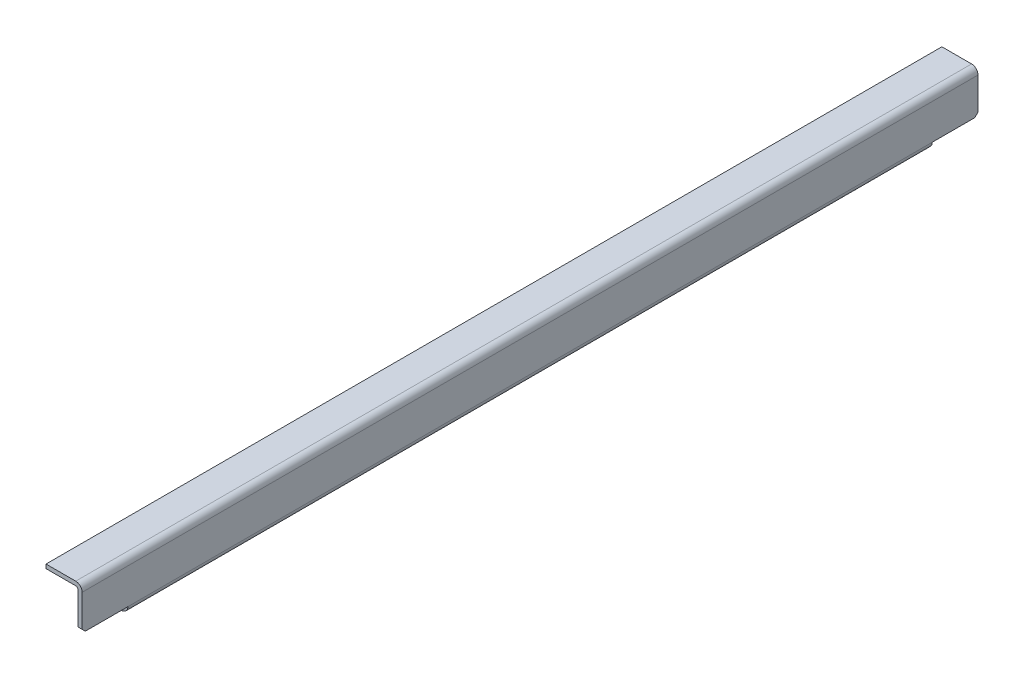
from build123d import *

# Parameters (mm, degrees)
BOSS_EXTRUDE1_DEPTH    = 1116
SKETCH2_W              = 92.475127077
SKETCH2_H              = 38.646657261
SKETCH2_W_2            = 90.397253408
SKETCH2_H_2            = 44.857464027
CUT_EXTRUDE1_DEPTH     = 1116
SKETCH3_R              = 4
CUT_EXTRUDE2_DEPTH     = 1116
M10_TAPPED_HOLE1_D     = 8.5
M10_TAPPED_HOLE1_DEPTH = 24.5
M10_TAPPED_HOLE1_TIP   = 2.553657631
CHAMFER1_SIZE          = 4


with BuildPart() as part:
    # Sketch1 → Boss-Extrude1 (new body)
    with BuildSketch(Plane.XY):
        with BuildLine():
            Line((0, 0), (37, 0))
            ThreePointArc((37, 0), (42.656854249, -2.343145751), (45, -8))
            Line((45, -8), (45, -52))
            ThreePointArc((45, -52), (42.656854249, -57.656854249), (37, -60))
            Line((37, -60), (0, -60))
            Line((0, -60), (0, -55))
            Line((0, -55), (37, -55))
            ThreePointArc((37, -55), (39.121320344, -54.121320344), (40, -52))
            Line((40, -52), (40, -8))
            ThreePointArc((40, -8), (39.121320344, -5.878679656), (37, -5))
            Line((37, -5), (0, -5))
            Line((0, -5), (0, 0))
        make_face()
    extrude(amount=BOSS_EXTRUDE1_DEPTH)

    # Sketch2 → Cut-Extrude1 (cut)
    with BuildSketch(Plane.ZY):
        with Locations((1105.237563539, -71.323328631)):
            Rectangle(SKETCH2_W, SKETCH2_H)
        with Locations((11.801373296, -74.428732013)):
            Rectangle(SKETCH2_W_2, SKETCH2_H_2)
    extrude(amount=-CUT_EXTRUDE1_DEPTH, mode=Mode.SUBTRACT)

    # Sketch3 → Cut-Extrude2 (cut)
    with BuildSketch(Plane(origin=(0, -55, 0), x_dir=(1, 0, 0), z_dir=(0, 1, 0))):
        with Locations(Location((12.5, -92, 0), (0, 0, 270))):
            Circle(SKETCH3_R)
    extrude(amount=-CUT_EXTRUDE2_DEPTH, mode=Mode.SUBTRACT)

    # M10 Tapped Hole1
    with Locations(Plane(origin=(0, -55, 0), x_dir=(1, 0, 0), z_dir=(0, 1, 0))):
        with Locations((12.5, -92)):
            Hole(M10_TAPPED_HOLE1_D / 2, depth=M10_TAPPED_HOLE1_DEPTH)
            with Locations((0, 0, -(M10_TAPPED_HOLE1_DEPTH + M10_TAPPED_HOLE1_TIP / 2))):  # 118° drill point
                Cone(0, M10_TAPPED_HOLE1_D / 2, M10_TAPPED_HOLE1_TIP, mode=Mode.SUBTRACT)

    # Chamfer1
    chamfer1_edges = [part.edges().sort_by_distance(p)[0] for p in [
        (42.5, -52, 0),
        (42.5, -52, 1116),
    ]]
    chamfer(chamfer1_edges, length=CHAMFER1_SIZE)


solid = part.part
